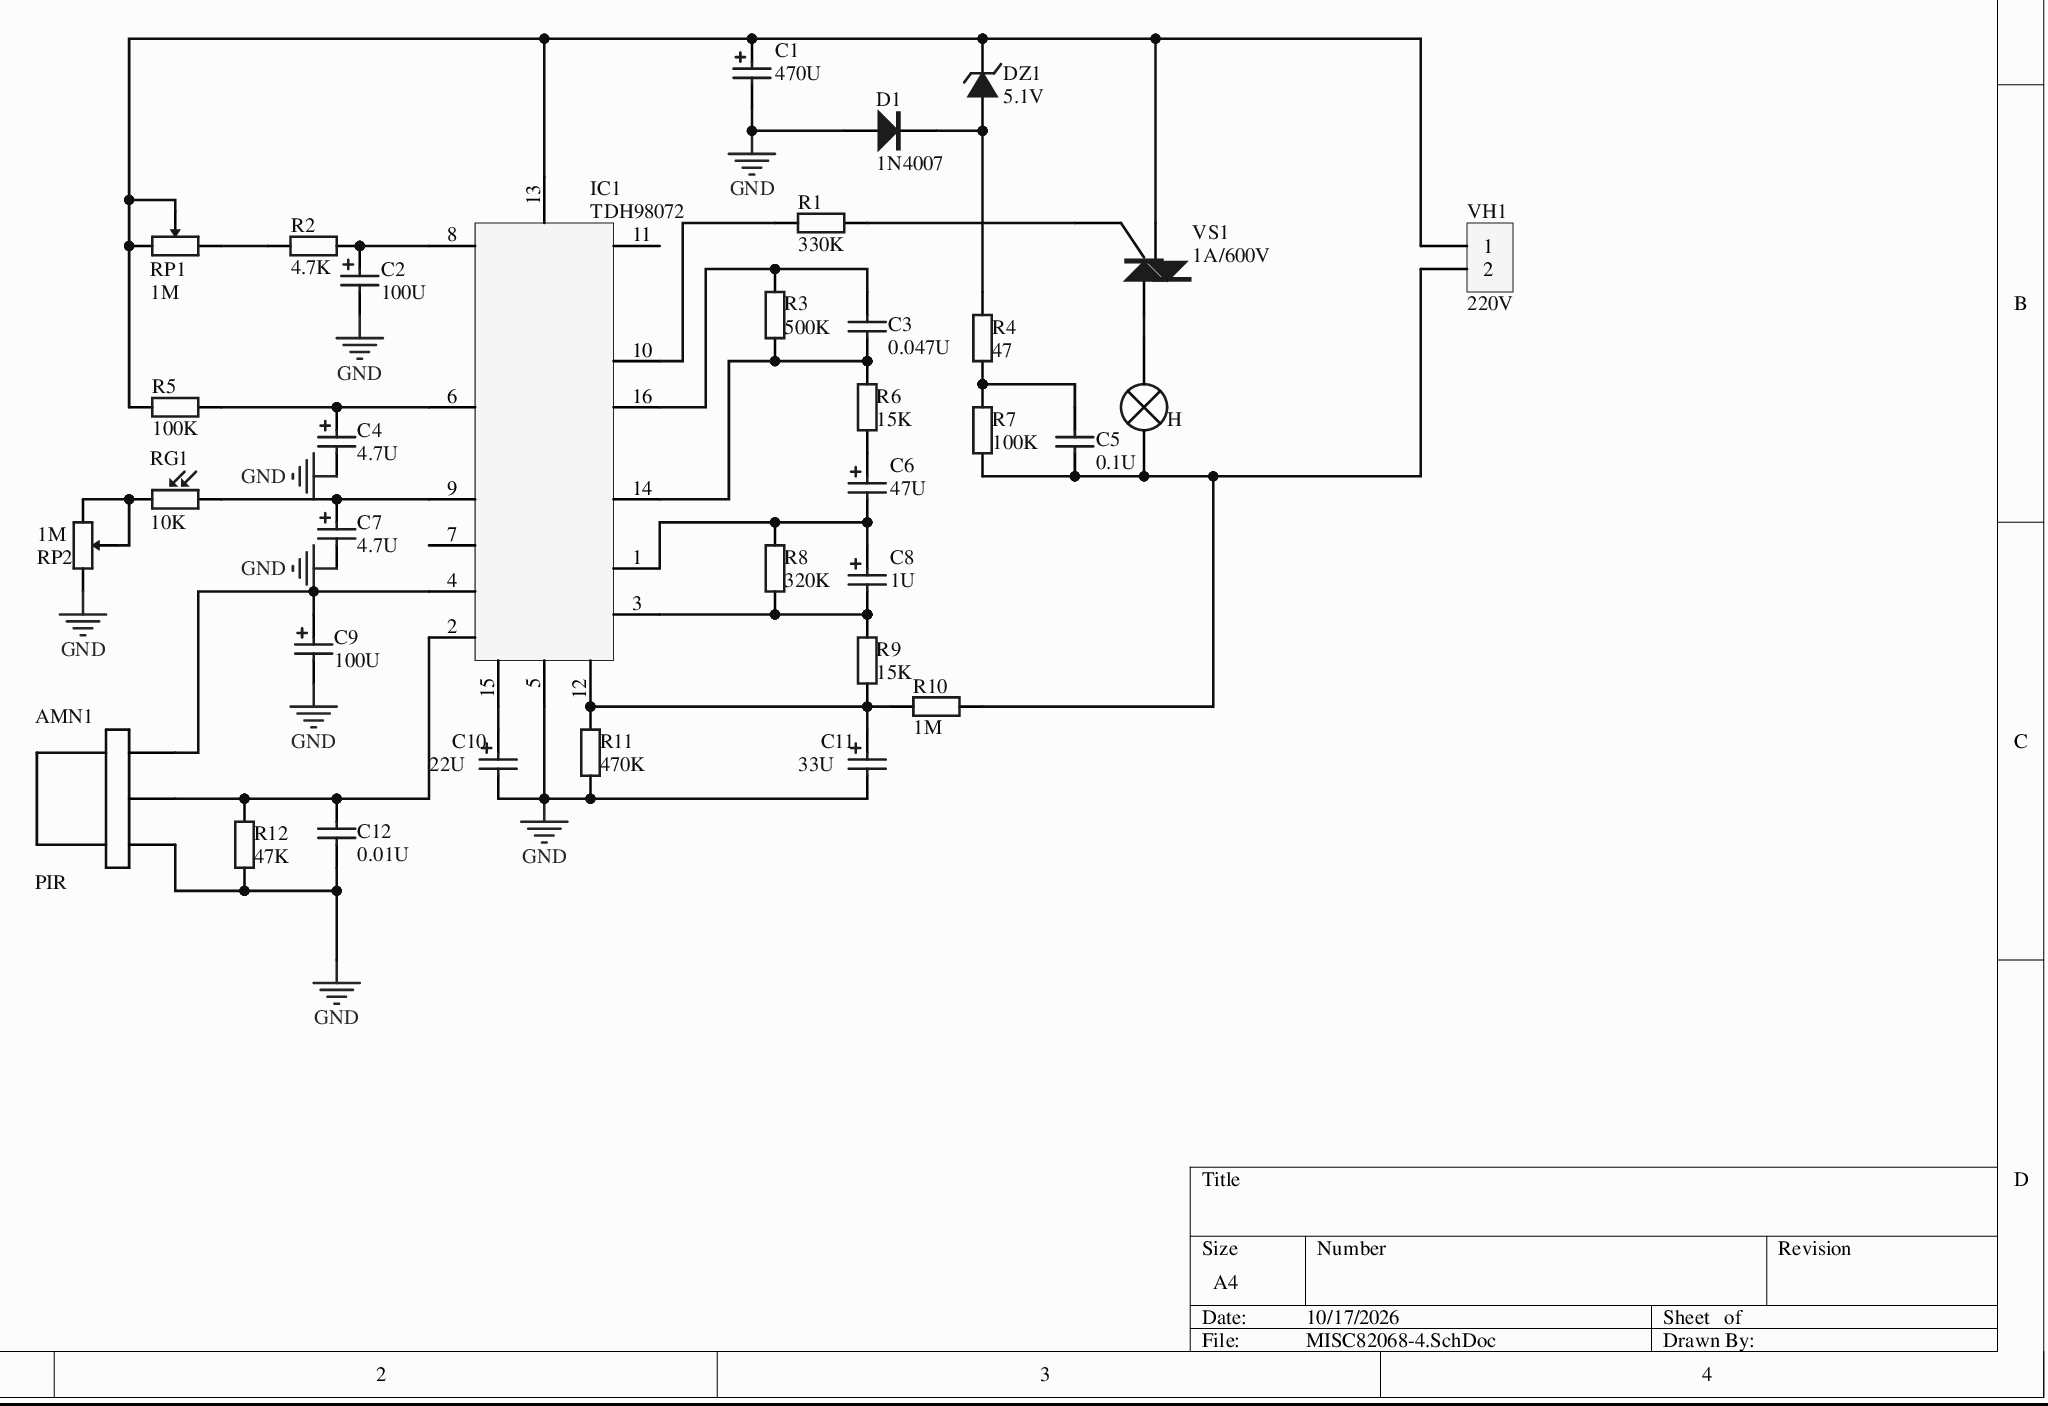
[diagram p0: MISC82068-4.SchDoc]
# Altium project MISC82068-5.PrjPcb
1 sheet, 34 parts. Net scope: global (net labels, ports and power ports of the same name join across sheets).
Board file: MISC82068.PcbDoc

## Sheet MISC82068-4.SchDoc
size A4

### Parts
*1  H  [HDR1X2]
AMN1  PIR  [HDR1X3]
C1  470U  [POLAR0.8]
C2  100U  [POLAR0.8]
C3  0.047U  [RAD-0.3]
C4  4.7U  [POLAR0.8]
C5  0.1U  [RAD-0.3]
C6  47U  [POLAR0.8]
C7  4.7U  [POLAR0.8]
C8  1U  [POLAR0.8]
C9  100U  [POLAR0.8]
C10  22U  [POLAR0.8]
C11  33U  [POLAR0.8]
C12  0.01U  [RAD-0.3]
D1  1N4007  [DO-41]
DZ1  5.1V  [DO-35]
IC1  TDH98072  [DIP16]
R1  330K  [AXIAL-0.4]
R2  4.7K  [AXIAL-0.4]
R3  500K  [AXIAL-0.4]
R4  47  [AXIAL-0.4]
R5  100K  [AXIAL-0.4]
R6  15K  [AXIAL-0.4]
R7  100K  [AXIAL-0.4]
R8  320K  [AXIAL-0.4]
R9  15K  [AXIAL-0.4]
R10  1M  [AXIAL-0.4]
R11  470K  [AXIAL-0.4]
R12  47K  [AXIAL-0.4]
RG1  10K  [AXIAL-0.4]
RP1  1M  [3296W]
RP2  1M  [3296W]
VH1  220V  [VH3.96-2A]
VS1  1A/600V  [LED 3mm-2P]

### Nets
GND: AMN1.3 C1.2 C2.2 C4.2 C7.2 C9.2 C10.2 C11.2 C12.1 D1.1(A) IC1.5(VSS) R11.1 R12.1 RP2.3
Net*1_1: *1.1 VS1.1
Net*1_2: *1.2 C5.1 R7.1 R10.2 VH1.2
NetAMN1_1: AMN1.1 C9.1 IC1.4(VSS)
NetAMN1_2: AMN1.2 C12.2 IC1.2(VSS) R12.2
NetC1_1: C1.1 DZ1.2(K) IC1.13(VSS) R5.1 RP1.1 RP1.2 VH1.1 VS1.2
NetC2_1: C2.1 IC1.8(VSS) R2.2
NetC3_1: C3.1 IC1.14(VSS) R3.1 R6.2
NetC3_2: C3.2 IC1.16(VSS) R3.2
NetC4_1: C4.1 IC1.6(VSS) R5.2
NetC5_2: C5.2 R4.1 R7.2
NetC6_1: C6.1 R6.1
NetC6_2: C6.2 C8.1 IC1.1(VSS) R8.2
NetC7_1: C7.1 IC1.9(VSS) RG1.1
NetC8_2: C8.2 IC1.3(VSS) R8.1 R9.2
NetC10_1: C10.1 IC1.15(VSS)
NetC11_1: C11.1 IC1.12(VSS) R9.1 R10.1 R11.2
NetD1_2: D1.2(K) DZ1.1(A) R4.2
NetIC1_10: IC1.10(VSS) R1.2
NetR1_1: R1.1 VS1.3
NetR2_1: R2.1 RP1.3
NetRG1_2: RG1.2 RP2.1 RP2.2

Not connected (* = marked no-connect by the designer): IC1 7(VSS)* 11(VSS)*

### Library data of the parts
C1 C2 C4 C6-C11 = Cap Pol2: Polarized Capacitor (Axial); Value: 100pF; Published: 8-Jun-2000; LatestRevisionDate: 17-Jul-2002; LatestRevisionNote: Re-released for DXP Platform.; PackageReference: POLAR0.8; PackageDescription: Polarized Capacitor; 2 Leads; Publisher: Altium Limited
C3 C5 C12 = Cap: Capacitor; Value: 100pF; Published: 8-Jun-2000; LatestRevisionDate: 17-Jul-2002; LatestRevisionNote: Re-released for DXP Platform.; PackageReference: RAD-0.3; PackageDescription: Radial Cap, Thru-Hole; 2 Leads; 0.3 in Pin Spacing; Publisher: Altium Limited
D1 = 1N4007: Rectifier diode; BOM名称: Rectifier diode
DZ1 = 1N4619: 3V/0.5W Zener diode; BOM名称: 3V/0.5W Zener diode
R1-R12 = Res2: Resistor; Value: 1K; Published: 8-Jun-2000; LatestRevisionDate: 17-Jul-2002; LatestRevisionNote: Re-released for DXP Platform.; PackageReference: AXIAL-0.4; PackageDescription: Axial Device, Thru-Hole; 2 Leads; 0.4 in Pin Spacing; Publisher: Altium Limited
RG1 = RG: Photoresistor; BOM名称: Photoresistor
RP1 RP2 = RP: Single potentiometer; BOM名称: Through-hole potentiometer
VH1 = VH2
VS1 = 1A/600V: BOM名称: Rectifier diode